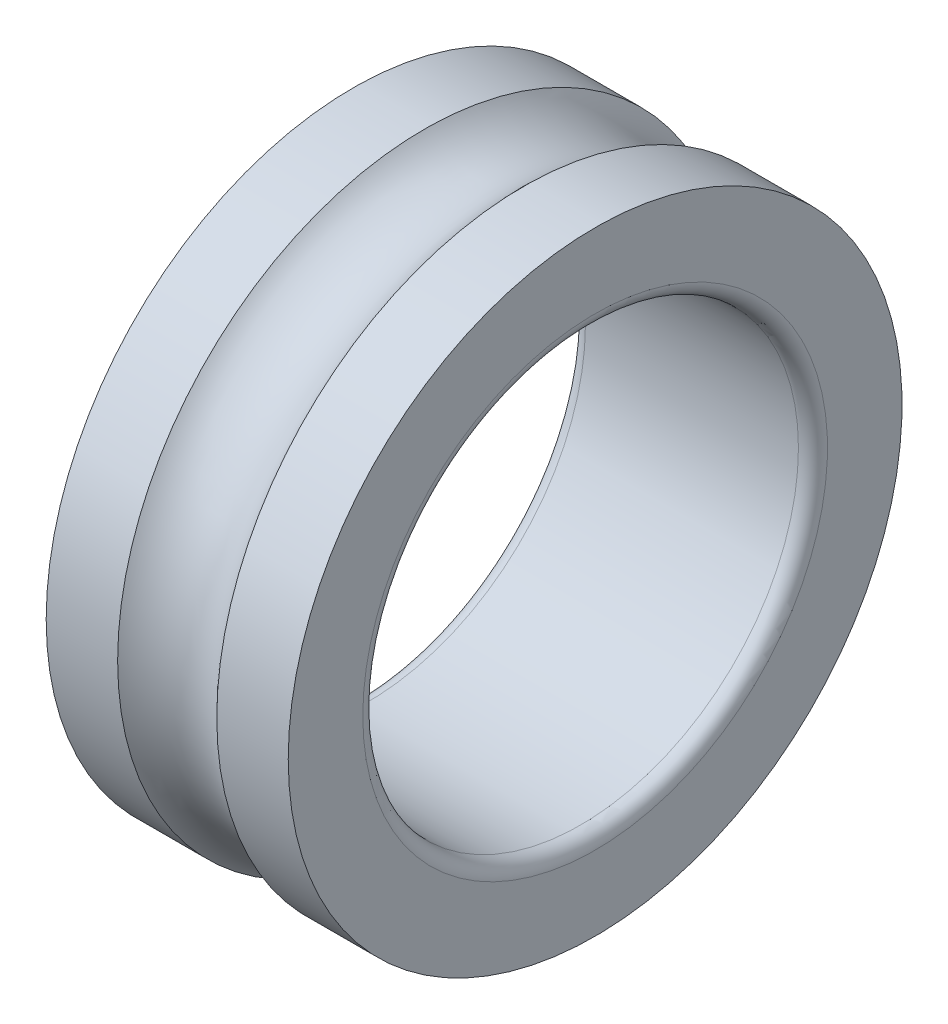
SolidWorks part; units mm, degrees
ref_plane "Front Plane" through (0, 0, 0) normal (0, 0, 1) x (1, 0, 0)
ref_plane "Top Plane" through (0, 0, 0) normal (0, 1, 0) x (1, 0, 0)
ref_plane "Right Plane" through (0, 0, 0) normal (1, 0, 0) x (0, 0, -1)
other "Configuration Table"
sketch "Sketch1" plane through (0, 0, 0) normal (0, 0, 1) x (1, 0, 0)
  line L0 (0, -8.205) -> (0, 34.7674) construction
  line L1 (-18.9193, 0) -> (23.8716, 0) construction
  line L2 (5.1205, 31.7) -> (12.5, 31.7)
  line L3 (-12.5, 22.5) -> (12.5, 22.5)
  line L4 (-12.5, 22.5) -> (-12.5, 31.7)
  line L5 (-12.5, 31.7) -> (-5.1205, 31.7)
  line L6 (12.5, 22.5) -> (12.5, 31.7)
  line L7 (-12.5, 22.5) -> (12.5, 31.7) construction
  line L8 (-12.5, 31.7) -> (12.5, 22.5) construction
  arc A0 (-5.1205, 31.7) -> (5.1205, 31.7) centre (0, 36.25) ccw
  point P5 (0, 27.1)
  dimension "D3" = 13.7
  dimension "D1" = 9.2
  dimension "D2" = 25
  dimension "D4" = 22.5
  dimension "D5" = 36.25
revolve "Revolve1" add sketch "Sketch1" angle 360 about L1
fillet "Fillet1" radius 1.5 2 edges at (-12.5, 0, 22.5) (12.5, 0, 22.5)
